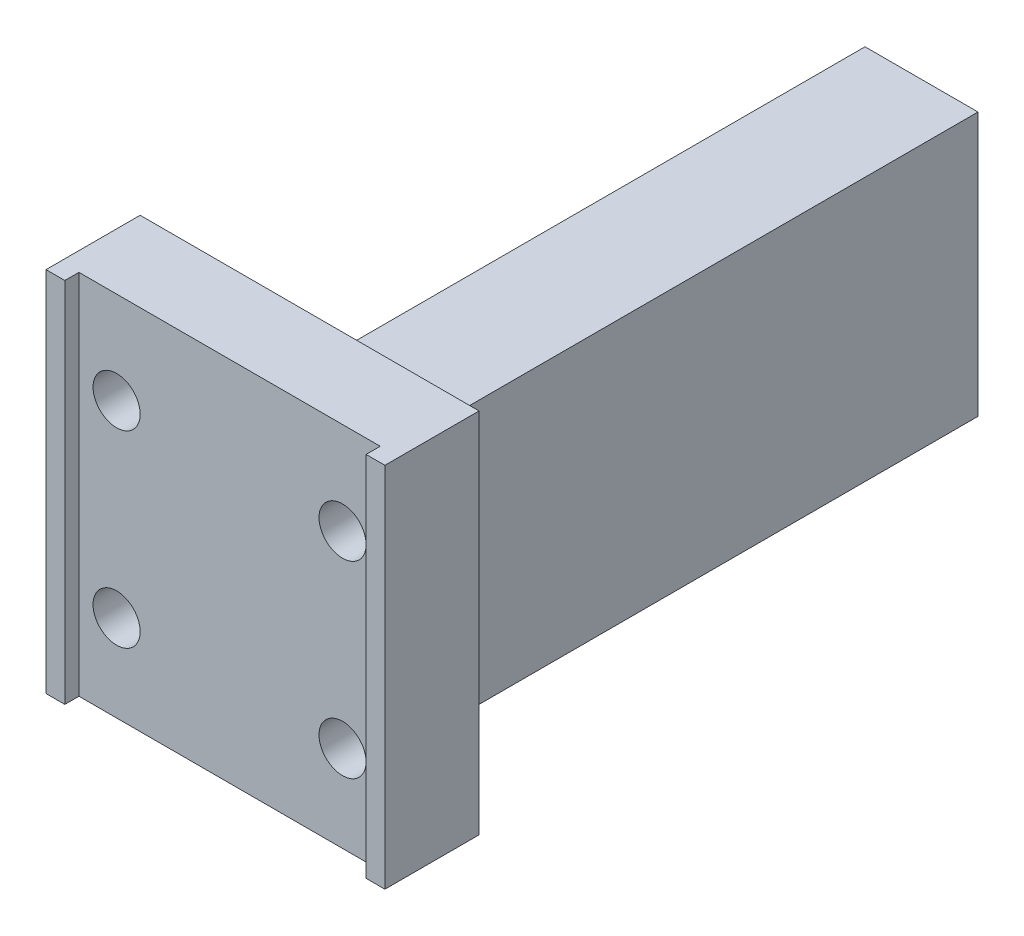
from build123d import *

# Parameters (mm, degrees)
SKETCH_1_W                = 36
SKETCH_1_H                = 39
EXTRUDE_1_DEPTH           = 10
SKETCH_2_W                = 32
SKETCH_2_H                = 39
CUT_EXTRUDE_1_DEPTH       = 1.5
SKETCH_3_W                = 12
SKETCH_3_H                = 28
EXTRUDE_2_DEPTH           = 65
HOLE_WIZARD_5_0_5_1_D     = 5
HOLE_WIZARD_5_0_5_1_DEPTH = 10


with BuildPart() as part:
    # 草图1 → 凸台-拉伸1 (new body)
    with BuildSketch(Plane.XY):
        Rectangle(SKETCH_1_W, SKETCH_1_H)
    extrude(amount=EXTRUDE_1_DEPTH)

    # 草图2 → 切除-拉伸1 (cut)
    with BuildSketch(Plane.XY.offset(10)):
        Rectangle(SKETCH_2_W, SKETCH_2_H)
    extrude(amount=-CUT_EXTRUDE_1_DEPTH, mode=Mode.SUBTRACT)

    # 草图3 → 凸台-拉伸2 (add)
    with BuildSketch(Plane(origin=(0, 0, 0), x_dir=(-1, 0, 0), z_dir=(0, 0, -1))):
        with Locations((0, -5.5)):
            Rectangle(SKETCH_3_W, SKETCH_3_H)
    extrude(amount=EXTRUDE_2_DEPTH)

    # Ø5.0 (5) 直径孔1
    with Locations(Plane(origin=(0, 0, 0), x_dir=(-1, 0, 0), z_dir=(0, 0, -1))):
        with Locations((-12, 9.7), (12, 9.7), (12, -10.3), (-12, -10.3)):
            Hole(HOLE_WIZARD_5_0_5_1_D / 2, depth=HOLE_WIZARD_5_0_5_1_DEPTH)


solid = part.part
